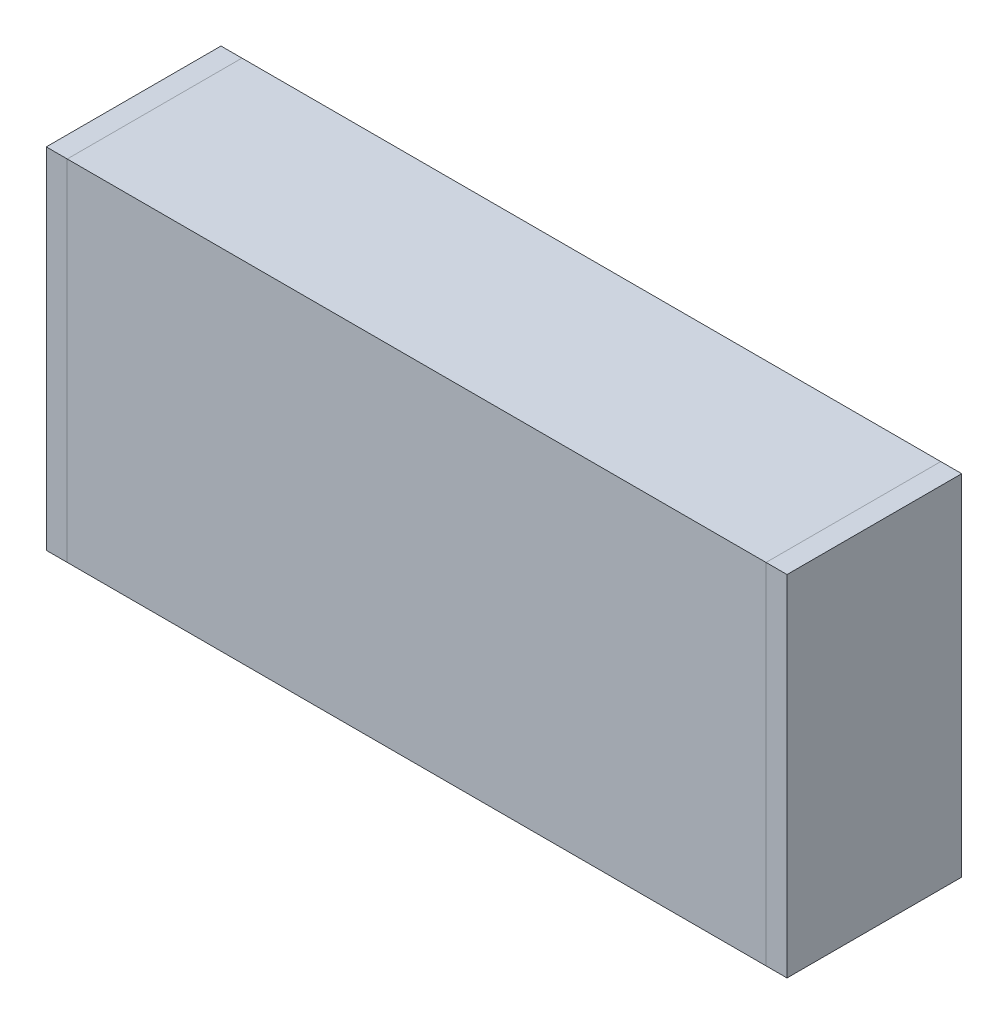
from build123d import *

# Parameters (mm, degrees)
C_CHANNEL_C80X40X15X1_5_1_DEPTH = 200
SKETCH12_W                      = 50
SKETCH12_H                      = 100
BOSS_EXTRUDE1_DEPTH             = 6
SKETCH13_W                      = 50
SKETCH13_H                      = 100
BOSS_EXTRUDE2_DEPTH             = 6
SKETCH14_R                      = 6
CUT_EXTRUDE1_DEPTH              = 14


with BuildPart() as part:
    # Sketch11 → C-channel C80X40X15X1.5(1) (new body)
    with BuildSketch(Plane(origin=(0, 0, 0), x_dir=(0, 0, -1), z_dir=(1, 0, 0))):
        Polygon((0, -50), (0, 50), (50, 50), (50, 35), (48.5, 35), (48.5, 48.5), (1.5, 48.5), (1.5, -48.5), (48.5, -48.5), (48.5, -35), (50, -35), (50, -50), align=None)
    extrude(amount=C_CHANNEL_C80X40X15X1_5_1_DEPTH)


with BuildPart() as body_2:
    # Sketch12 → Boss-Extrude1 (new body)
    with BuildSketch(Plane(origin=(200, 0, 0), x_dir=(0, 0, -1), z_dir=(1, 0, 0))):
        with Locations((25, 0)):
            Rectangle(SKETCH12_W, SKETCH12_H)
    extrude(amount=BOSS_EXTRUDE1_DEPTH)


with BuildPart() as body_3:
    # Sketch13 → Boss-Extrude2 (new body)
    with BuildSketch(Plane.ZY):
        with Locations((-25, 0)):
            Rectangle(SKETCH13_W, SKETCH13_H)
    extrude(amount=BOSS_EXTRUDE2_DEPTH)

    # Sketch14 → Cut-Extrude1 (cut)
    with BuildSketch(Plane.ZY.offset(6)):
        with Locations((-35, 0)):
            Circle(SKETCH14_R)
    extrude(amount=-CUT_EXTRUDE1_DEPTH, mode=Mode.SUBTRACT)


solid = Compound([part.part, body_2.part, body_3.part])
